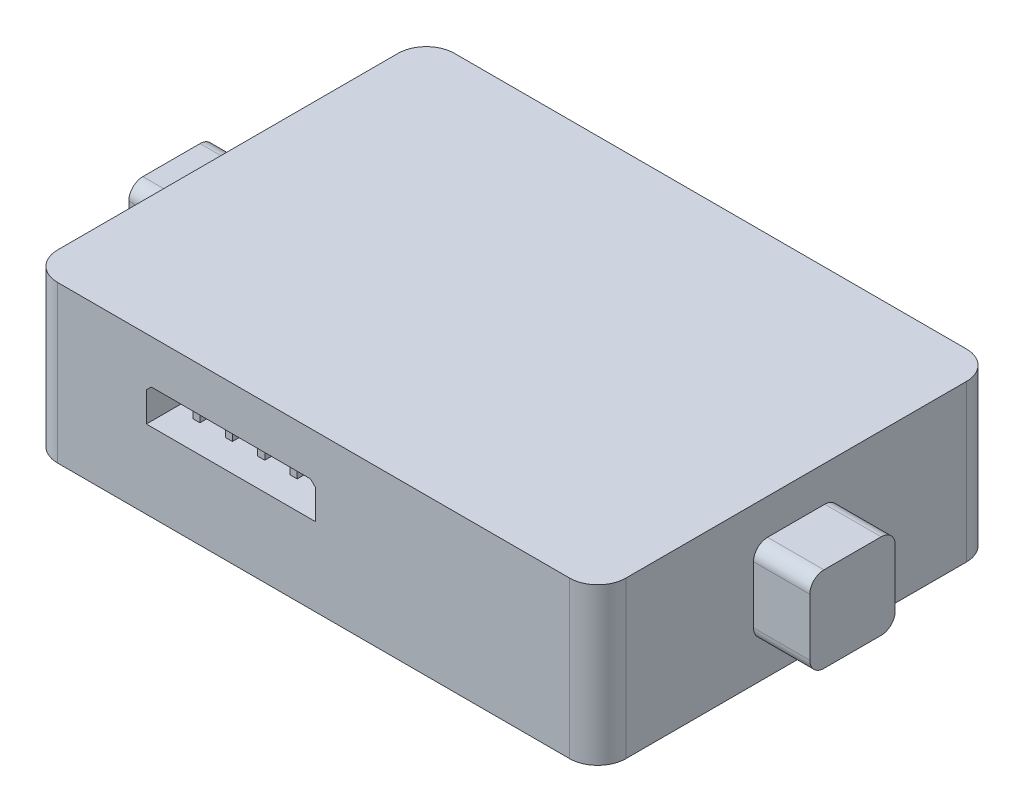
SolidWorks part; units mm, degrees
ref_plane "前视基准面" through (0, 0, 0) normal (0, 0, 1) x (1, 0, 0)
ref_plane "上视基准面" through (0, 0, 0) normal (0, 1, 0) x (1, 0, 0)
ref_plane "右视基准面" through (0, 0, 0) normal (1, 0, 0) x (0, 0, -1)
ref_plane "基准面4" through (0, 11.1, 0) normal (0, 1, 0) x (1, 0, 0)
sketch "草图1" plane through (0, 11.1, 0) normal (0, 1, 0) x (1, 0, 0)
  line L0 (-20.165, 14.08) -> (-20.165, -14.08)
  line L1 (-20.165, -14.08) -> (20.165, -14.08)
  line L2 (20.165, -14.08) -> (20.165, 14.08)
  line L3 (20.165, 14.08) -> (-20.165, 14.08)
extrude "凸台-拉伸1" add sketch "草图1" against normal blind 11.1
sketch "草图2" plane through (0, 0, 14.08) normal (0, 0, 1) x (1, 0, 0)
  line L0 (-11.865, 5.55) -> (0.135, 5.55)
  line L1 (0.135, 5.55) -> (0.135, 8)
  line L2 (0.135, 8) -> (-11.865, 8)
  line L3 (-11.865, 8) -> (-11.865, 5.55)
extrude "切除-拉伸1" cut sketch "草图2" against normal blind 10
sketch "草图3" plane through (0, 0, 4.08) normal (0, 0, 1) x (1, 0, 0)
  line L0 (-4.465, 7.025) -> (-4.465, 6.525)
  line L1 (-4.465, 6.525) -> (-4.965, 6.525)
  line L2 (-4.965, 6.525) -> (-4.965, 7.025)
  line L3 (-4.965, 7.025) -> (-4.465, 7.025)
extrude "凸台-拉伸2" add sketch "草图3" along normal blind 9
sketch "草图4" plane through (0, 0, 4.08) normal (0, 0, 1) x (1, 0, 0)
  line L0 (-9.565, 7.025) -> (-9.065, 7.025)
  line L1 (-9.065, 7.025) -> (-9.065, 6.525)
  line L2 (-9.065, 6.525) -> (-9.565, 6.525)
  line L3 (-9.565, 6.525) -> (-9.565, 7.025)
extrude "凸台-拉伸3" add sketch "草图4" along normal blind 9
sketch "草图5" plane through (0, 0, 4.08) normal (0, 0, 1) x (1, 0, 0)
  line L0 (-7.265, 7.025) -> (-6.765, 7.025)
  line L1 (-6.765, 7.025) -> (-6.765, 6.525)
  line L2 (-6.765, 6.525) -> (-7.265, 6.525)
  line L3 (-7.265, 6.525) -> (-7.265, 7.025)
extrude "凸台-拉伸4" add sketch "草图5" along normal blind 9
sketch "草图6" plane through (0, 0, 4.08) normal (0, 0, 1) x (1, 0, 0)
  line L0 (-2.165, 7.025) -> (-2.165, 6.525)
  line L1 (-2.165, 6.525) -> (-2.665, 6.525)
  line L2 (-2.665, 6.525) -> (-2.665, 7.025)
  line L3 (-2.665, 7.025) -> (-2.165, 7.025)
extrude "凸台-拉伸5" add sketch "草图6" along normal blind 9
sketch "草图7" plane through (-20.165, 0, 0) normal (-1, 0, 0) x (0, 0, 1)
  line L0 (-3.03, 2.52) -> (-3.03, 8.58)
  line L1 (-3.03, 8.58) -> (3.03, 8.58)
  line L2 (3.03, 8.58) -> (3.03, 2.52)
  line L3 (3.03, 2.52) -> (-3.03, 2.52)
extrude "凸台-拉伸6" add sketch "草图7" along normal blind 4
sketch "草图8" plane through (20.165, 0, 0) normal (1, 0, 0) x (0, 0, -1)
  line L0 (-3.03, 2.52) -> (-3.03, 8.58)
  line L1 (-3.03, 8.58) -> (3.03, 8.58)
  line L2 (3.03, 8.58) -> (3.03, 2.52)
  line L3 (3.03, 2.52) -> (-3.03, 2.52)
extrude "凸台-拉伸7" add sketch "草图8" along normal blind 4
chamfer "倒角1" distance 0.35 angle 45 2 edges at (0.135, 8, 9.08) (-11.865, 8, 9.08)
fillet "圆角1" radius 1 8 edges at (22.165, 8.58, -3.03) (-22.165, 8.58, -3.03) (-22.165, 8.58, 3.03) (-22.165, 2.52, -3.03) (22.165, 2.52, -3.03) (-22.165, 2.52, 3.03) (22.165, 2.52, 3.03) (22.165, 8.58, 3.03)
fillet "圆角2" radius 2 4 edges at (20.165, 5.55, -14.08) (20.165, 5.55, 14.08) (-20.165, 5.55, -14.08) (-20.165, 5.55, 14.08)
